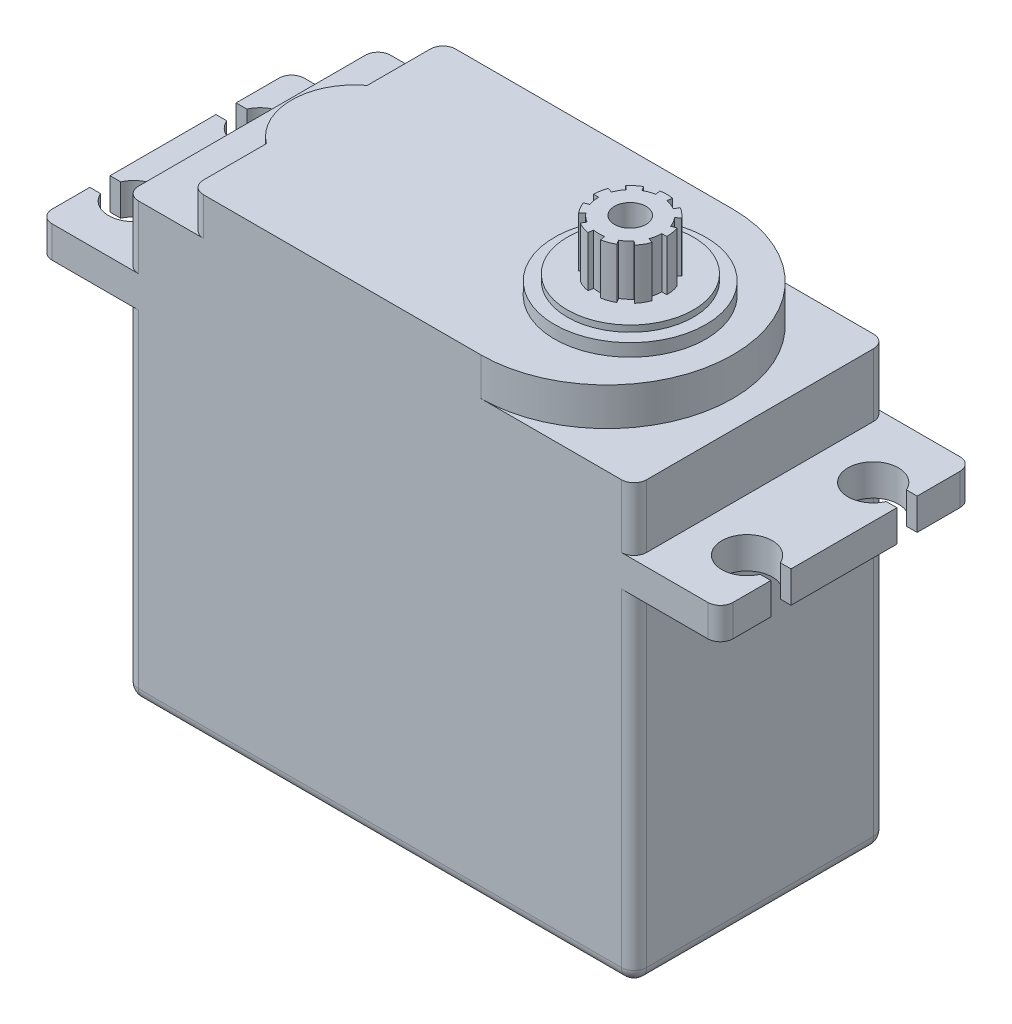
SolidWorks part; units mm, degrees
ref_plane "Front Plane" through (0, 0, 0) normal (0, 0, 1) x (1, 0, 0)
ref_plane "Top Plane" through (0, 0, 0) normal (0, 1, 0) x (1, 0, 0)
ref_plane "Right Plane" through (0, 0, 0) normal (1, 0, 0) x (0, 0, -1)
sketch "Sketch1" plane through (0, 0, 0) normal (0, 0, 1) x (1, 0, 0)
  line L0 (0, 0) -> (-50000, 0) construction
  line L1 (0, 0) -> (0, 50000) construction
  line L2 (20.15, 8) -> (27, 8)
  line L3 (-20.15, 18.5) -> (20.15, 18.5)
  line L4 (-20.15, 18.5) -> (-20.15, 10.5)
  line L5 (-20.15, -19) -> (20.15, -19)
  line L6 (20.15, 18.5) -> (20.15, 10.5)
  line L7 (-27, 10.5) -> (-20.15, 10.5)
  line L8 (-27, 10.5) -> (-27, 8)
  line L9 (-27, 8) -> (-20.15, 8)
  line L10 (27, 10.5) -> (27, 8)
  line L11 (20.15, 10.5) -> (27, 10.5)
  line L12 (20.15, 8) -> (20.15, -19)
  line L13 (-20.15, 8) -> (-20.15, -19)
  dimension "D1" = 8
  dimension "D2" = 6.85
  dimension "D3" = 2.5
  dimension "D4" = 40.3
  dimension "D5" = 27
  dimension "D6" = 54
  dimension "D7" = 20.15
extrude "Boss-Extrude1" add sketch "Sketch1" along normal blind 20
fillet "Fillet1" radius 1 18 edges at (-20.15, 14.5, 20) (20.15, 14.5, 20) (20.15, 18.5, 10) (-20.15, 18.5, 10) (20.15, 14.5, 0) (-20.15, 14.5, 0) (-20.15, -19, 10) (0, -19, 20) (20.15, -19, 10) (0, -19, 0) (-20.15, -5.5, 0) (20.15, -5.5, 0) (20.15, -5.5, 20) (-20.15, -5.5, 20) (27, 9.25, 0) (27, 9.25, 20) (-27, 9.25, 0) (-27, 9.25, 20)
sketch "Sketch2" plane through (0, 10.5, 0) normal (0, 1, 0) x (1, 0, 0)
  line L0 (-0.1717, -10.2) -> (49999.8283, -10.2) construction
  line L1 (0, 0) -> (0, -50000) construction
  line L2 (-26.148, -4.4) -> (-29.2227, -4.4)
  line L3 (-24.315, -5.2) -> (-30.8838, -5.2) construction
  line L4 (-24, -15) -> (-30.5688, -15) construction
  line L5 (-29.2227, -4.4) -> (-29.2227, -6)
  line L6 (-26.148, -6) -> (-29.2227, -6)
  line L7 (-26.148, -14.4) -> (-29.2227, -14.4)
  line L8 (-29.2227, -16) -> (-29.2227, -14.4)
  line L9 (-26.148, -16) -> (-29.2227, -16)
  line L10 (26.148, -16) -> (29.2227, -16)
  line L11 (29.2227, -16) -> (29.2227, -14.4)
  line L12 (26.148, -14.4) -> (29.2227, -14.4)
  line L13 (29.2227, -4.4) -> (29.2227, -6)
  line L14 (26.148, -6) -> (29.2227, -6)
  line L15 (26.148, -4.4) -> (29.2227, -4.4)
  arc A0 (-26.148, -14.4) -> (-26.148, -16) centre (-24.315, -15.2) cw
  arc A1 (26.148, -14.4) -> (26.148, -16) centre (24.315, -15.2) ccw
  arc A2 (-26.148, -6) -> (-26.148, -4.4) centre (-24.315, -5.2) ccw
  arc A3 (26.148, -6) -> (26.148, -4.4) centre (24.315, -5.2) cw
  point P21 (-29.2227, -5.2)
  dimension "D2" = 10
  dimension "D1" = 48.63
  dimension "D3" = 2
extrude "Cut-Extrude1" cut sketch "Sketch2" against normal blind 20
sketch "Sketch3" plane through (0, 18.5, 0) normal (0, 1, 0) x (1, 0, 0)
  line L0 (-40.2617, -10) -> (49959.7383, -10) construction
  line L1 (-14, 0) -> (8, 0)
  line L2 (-15, -1) -> (-15, -6)
  line L3 (-14, -20) -> (8, -20)
  line L4 (-15, -14) -> (-15, -19)
  line L5 (0, 0) -> (0, 50000) construction
  line L7 (-26.8677, 6.7729) -> (25, 6.7729)
  line L8 (-26.8677, 6.7729) -> (-26.8677, -28.4888)
  line L9 (-26.8677, -28.4888) -> (25, -28.4888)
  line L10 (25, 6.7729) -> (25, -28.4888)
  arc A0 (8, -20) -> (8, 0) centre (8, -10) ccw
  arc A1 (-15, -6) -> (-15, -14) centre (-12, -10) ccw
  arc A2 (-14, -20) -> (-15, -19) centre (-14, -19) cw
  arc A3 (-15, -1) -> (-14, 0) centre (-14, -1) cw
  dimension "D2" = 1
  dimension "D1" = 25
extrude "Cut-Extrude2" cut sketch "Sketch3" against normal blind 3
sketch "Sketch4" plane through (0, 18.5, 0) normal (0, 1, 0) x (1, 0, 0)
  line L0 (27, -14.4) -> (27, -6) construction
  circle A0 centre (9.85, -10) radius 6
  dimension "D1" = 17.15
extrude "Boss-Extrude2" add sketch "Sketch4" along normal blind 1
sketch "Sketch5" plane through (0, 19.5, 0) normal (0, 1, 0) x (1, 0, 0)
  line L0 (27, -14.4) -> (27, -6) construction
  circle A0 centre (9.8513, -9.9876) radius 5
  point P2 (27, -10.2)
  dimension "D1" = 17.15
extrude "Boss-Extrude3" add sketch "Sketch5" along normal blind 0.5
sketch "Sketch6" plane through (0, 20, 0) normal (0, 1, 0) x (1, 0, 0)
  line L1 (10.2841, -7.538) -> (10.3536, -7.1441)
  line L3 (11.3, -7.4885) -> (11.1, -7.8349)
  line L5 (12.0715, -8.1359) -> (11.7651, -8.393)
  line L7 (12.5751, -9.0081) -> (12.1992, -9.1449)
  line L8 (6.95, -10) -> (7.35, -10)
  line L10 (7.5008, -9.1449) -> (7.1249, -9.0081)
  line L13 (8.6, -7.8349) -> (8.4, -7.4885)
  line L14 (7.9349, -8.393) -> (7.6285, -8.1359)
  line L15 (9.4159, -7.538) -> (9.3464, -7.1441)
  line L16 (9.4159, -12.462) -> (9.3464, -12.8559)
  line L19 (8.4, -12.5115) -> (8.6, -12.1651)
  line L20 (27, -14.4) -> (27, -6) construction
  line L21 (7.6285, -11.8641) -> (7.9349, -11.607)
  line L23 (7.1249, -10.9919) -> (7.5008, -10.8551)
  line L25 (12.1992, -10.8551) -> (12.5751, -10.9919)
  line L28 (11.1, -12.1651) -> (11.3, -12.5115)
  line L29 (10.2841, -12.462) -> (10.3536, -12.8559)
  line L30 (11.7651, -11.607) -> (12.0715, -11.8641)
  line L31 (12.35, -10) -> (12.75, -10)
  arc A0 (7.1249, -10.9919) -> (7.6285, -11.8641) centre (9.85, -10) ccw
  arc A1 (7.35, -10) -> (7.5008, -10.8551) centre (9.85, -10) ccw
  arc A2 (7.1249, -9.0081) -> (6.95, -10) centre (9.85, -10) ccw
  arc A3 (8.4, -7.4885) -> (7.6285, -8.1359) centre (9.85, -10) ccw
  arc A4 (10.3536, -7.1441) -> (9.3464, -7.1441) centre (9.85, -10) ccw
  arc A5 (12.0715, -8.1359) -> (11.3, -7.4885) centre (9.85, -10) ccw
  arc A6 (12.75, -10) -> (12.5751, -9.0081) centre (9.85, -10) ccw
  arc A7 (12.0715, -11.8641) -> (12.5751, -10.9919) centre (9.85, -10) ccw
  arc A8 (10.3536, -12.8559) -> (11.3, -12.5115) centre (9.85, -10) ccw
  arc A9 (8.4, -12.5115) -> (9.3464, -12.8559) centre (9.85, -10) ccw
  arc A10 (7.9349, -8.393) -> (7.5008, -9.1449) centre (9.85, -10) ccw
  arc A11 (9.4159, -7.538) -> (8.6, -7.8349) centre (9.85, -10) ccw
  arc A12 (11.1, -7.8349) -> (10.2841, -7.538) centre (9.85, -10) ccw
  arc A13 (12.1992, -9.1449) -> (11.7651, -8.393) centre (9.85, -10) ccw
  arc A14 (12.1992, -10.8551) -> (12.35, -10) centre (9.85, -10) ccw
  arc A15 (11.1, -12.1651) -> (11.7651, -11.607) centre (9.85, -10) ccw
  arc A16 (9.4159, -12.462) -> (10.2841, -12.462) centre (9.85, -10) ccw
  arc A17 (7.9349, -11.607) -> (8.6, -12.1651) centre (9.85, -10) ccw
  circle A18 centre (9.85, -10) radius 1
  dimension "D1" = 17.15
extrude "Boss-Extrude4" add sketch "Sketch6" along normal blind 4
hole_wizard "M3 Tapped Hole1" positions "3DSketch2" profile "Sketch8" tap size "M3" standard "GB"
sketch3d "3DSketch2"
  line L0 (9.85, 24, 10) -> (9.85, 20, 10) construction
  point P0 (9.85, 24, 10)
sketch "Sketch8" plane through (9.85, 24, 10) normal (1, 0, 0) x (0, 0, 1)
  line L0 (0, 0) -> (0, 8.2511)
  line L1 (0, 8.2511) -> (1.25, 7.5)
  line L2 (1.25, 7.5) -> (1.25, 0)
  line L5 (1.25, 0) -> (0, 0)
  line L10 (0, 8.2511) -> (-1.25, 7.5) construction
  line L11 (0, -6.35) -> (0, 107.95) construction
  dimension "螺纹孔钻头直径" = 2.5
  dimension "螺纹孔钻头深度" = 7.5
  dimension "导头角度" = 118
cosmetic thread "Cosmetic Thread1" parameters "D1"=6, "D2"=3
